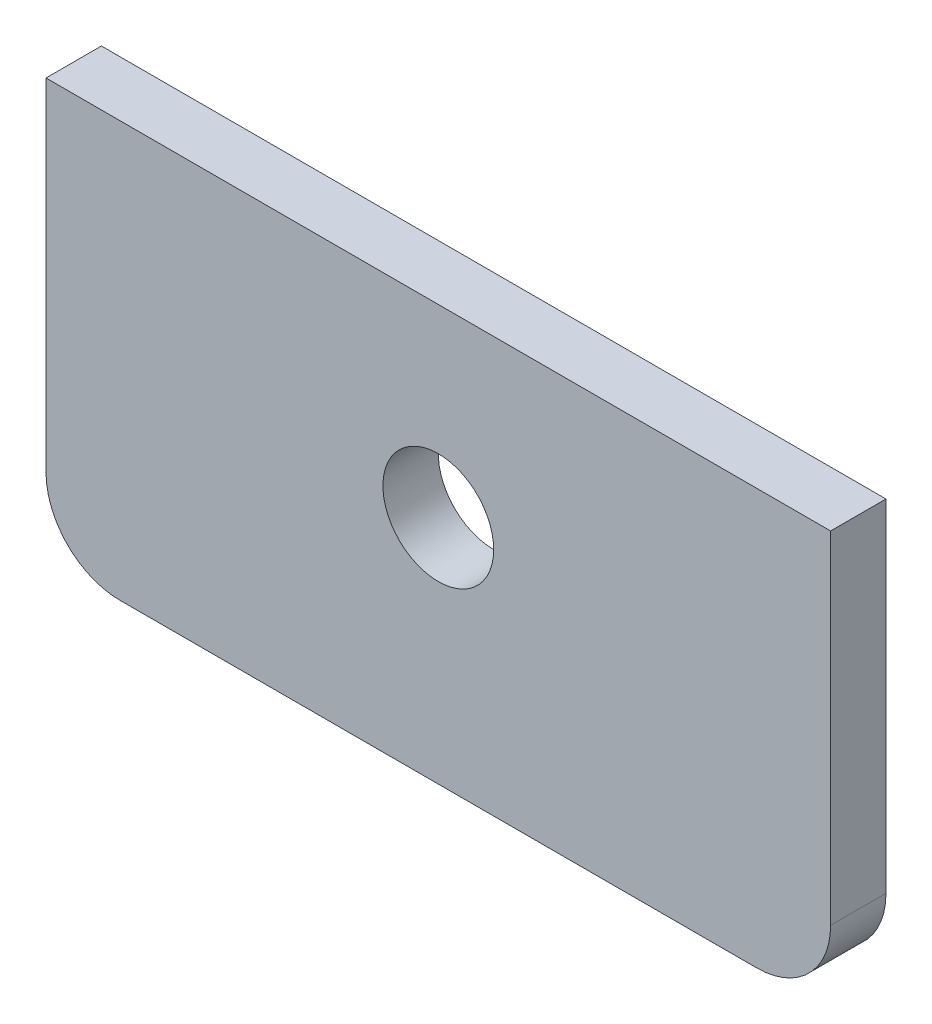
from build123d import *

# Parameters (mm, degrees)
SKETCH_1_R      = 6
EXTRUDE_1_DEPTH = 6


with BuildPart() as part:
    # 草图1 → 凸台-拉伸1 (new body)
    with BuildSketch(Plane.XY):
        with BuildLine():
            Line((-42.5, 22.5), (42.5, 22.5))
            Line((42.5, 22.5), (42.5, -14.5))
            ThreePointArc((42.5, -14.5), (40.156854249, -20.156854249), (34.5, -22.5))
            Line((34.5, -22.5), (-34.5, -22.5))
            ThreePointArc((-34.5, -22.5), (-40.156854249, -20.156854249), (-42.5, -14.5))
            Line((-42.5, -14.5), (-42.5, 22.5))
        make_face()
        with Locations((0, 2.5)):
            Circle(SKETCH_1_R, mode=Mode.SUBTRACT)
    extrude(amount=EXTRUDE_1_DEPTH)


solid = part.part
